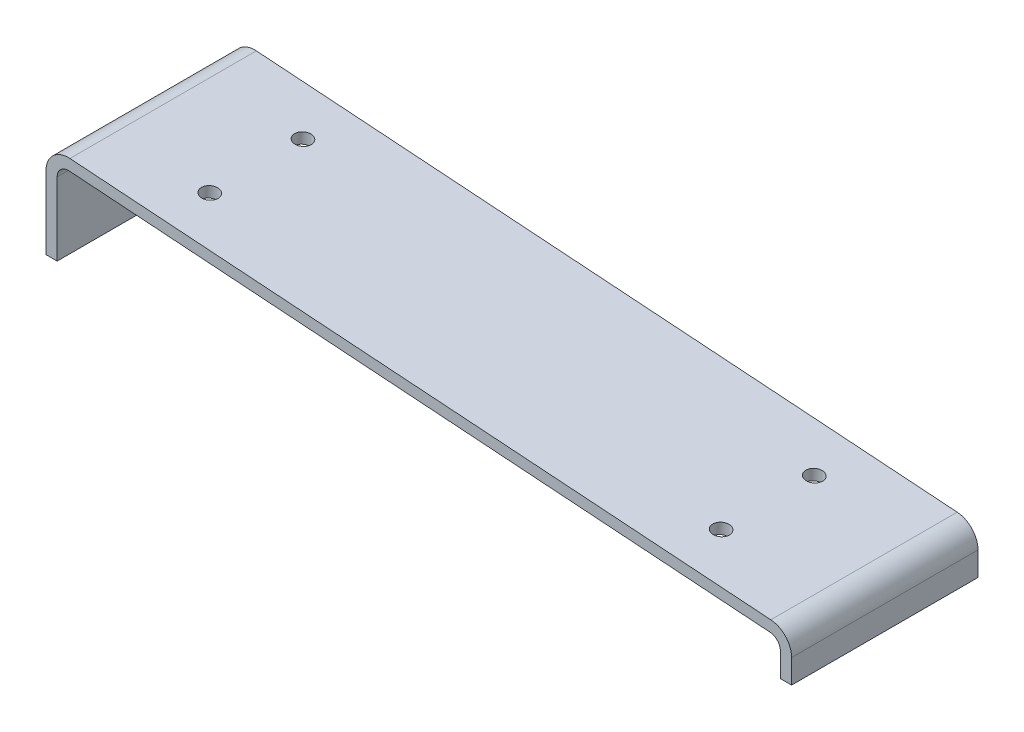
from build123d import *

# Parameters (mm, degrees)
BOSS_EXTRUDE1_DEPTH = 100
SKETCH4_R           = 4.5
CUT_EXTRUDE2_DEPTH  = 100
FILLET1_R           = 12
FILLET2_R           = 6


with BuildPart() as part:
    # Sketch1 → Boss-Extrude1 (new body)
    with BuildSketch(Plane.XY):
        Polygon((0, 0), (0, -52), (6, -52), (6, -6.434682036), (394, -33.594682036), (394, -52), (400, -52), (400, -28), align=None)
    extrude(amount=BOSS_EXTRUDE1_DEPTH)

    # Sketch4 → Cut-Extrude2 (cut)
    with BuildSketch(Plane(origin=(0, 0, 0), x_dir=(0.9975589671416267, -0.06982912769991385, 0), z_dir=(0.06982912769991385, 0.9975589671416267, 0))):
        with Locations(Location((63, -25, 0), (0, 0, 180))):
            Circle(SKETCH4_R)
        with Locations(Location((338, -25, 0), (0, 0, 180))):
            Circle(SKETCH4_R)
        with Locations(Location((63, -75, 0), (0, 0, 180))):
            Circle(SKETCH4_R)
        with Locations(Location((338, -75, 0), (0, 0, 180))):
            Circle(SKETCH4_R)
    extrude(amount=-CUT_EXTRUDE2_DEPTH, mode=Mode.SUBTRACT)

    # Fillet1
    fillet1_edges = [part.edges().sort_by_distance(p)[0] for p in [
        (400, -28, 50),
        (0, 0, 50),
    ]]
    fillet(fillet1_edges, radius=FILLET1_R)

    # Fillet2
    fillet2_edges = [part.edges().sort_by_distance(p)[0] for p in [
        (6, -6.434682036, 50),
        (394, -33.594682036, 50),
    ]]
    fillet(fillet2_edges, radius=FILLET2_R)


solid = part.part
